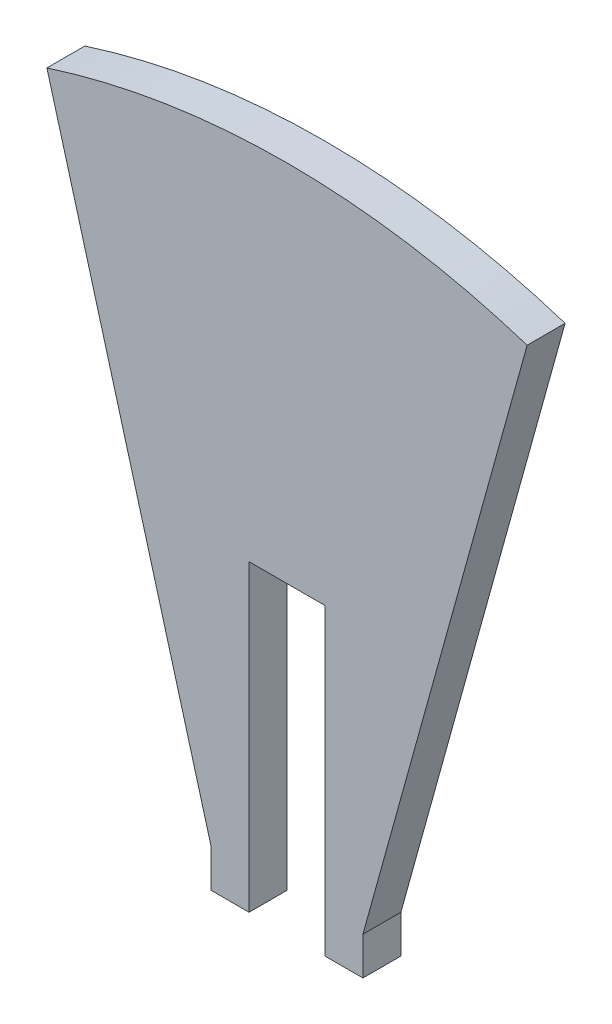
SolidWorks part; units mm, degrees
ref_plane "Front Plane" through (0, 0, 0) normal (0, 0, 1) x (1, 0, 0)
ref_plane "Top Plane" through (0, 0, 0) normal (0, 1, 0) x (1, 0, 0)
ref_plane "Right Plane" through (0, 0, 0) normal (1, 0, 0) x (0, 0, -1)
sketch "Sketch1" plane through (0, 0, 0) normal (0, 0, 1) x (1, 0, 0)
  line L0 (-63.2742, 196.0418) -> (-20, 40)
  line L1 (-20, 40) -> (-20, 30)
  line L2 (-20, 30) -> (20, 30)
  line L3 (20, 30) -> (20, 40)
  line L4 (20, 40) -> (63.2742, 196.0418)
  line L5 (0, 206) -> (0, 0) construction
  arc A0 (63.2742, 196.0418) -> (-63.2742, 196.0418) centre (0, 0) ccw
  dimension "D3" = 30
  dimension "D4" = 412
  dimension "D1" = 40
  dimension "D2" = 10
  dimension "D5" = 31
extrude "Boss-Extrude1" add sketch "Sketch1" along normal mid plane 10
sketch "Sketch2" plane through (0, 0, 5) normal (0, 0, 1) x (1, 0, 0)
  line L0 (-20, 30) -> (20, 30) construction
  line L1 (10, -50) -> (-10, -50)
  line L2 (10, -50) -> (10, 110)
  line L3 (10, 110) -> (-10, 110)
  line L4 (-10, -50) -> (-10, 110)
  line L5 (10, -50) -> (-10, 110) construction
  line L6 (10, 110) -> (-10, -50) construction
  point P0 (0, 30)
  dimension "D1" = 20
  dimension "D2" = 80
extrude "Cut-Extrude1" cut sketch "Sketch2" against normal blind 10
